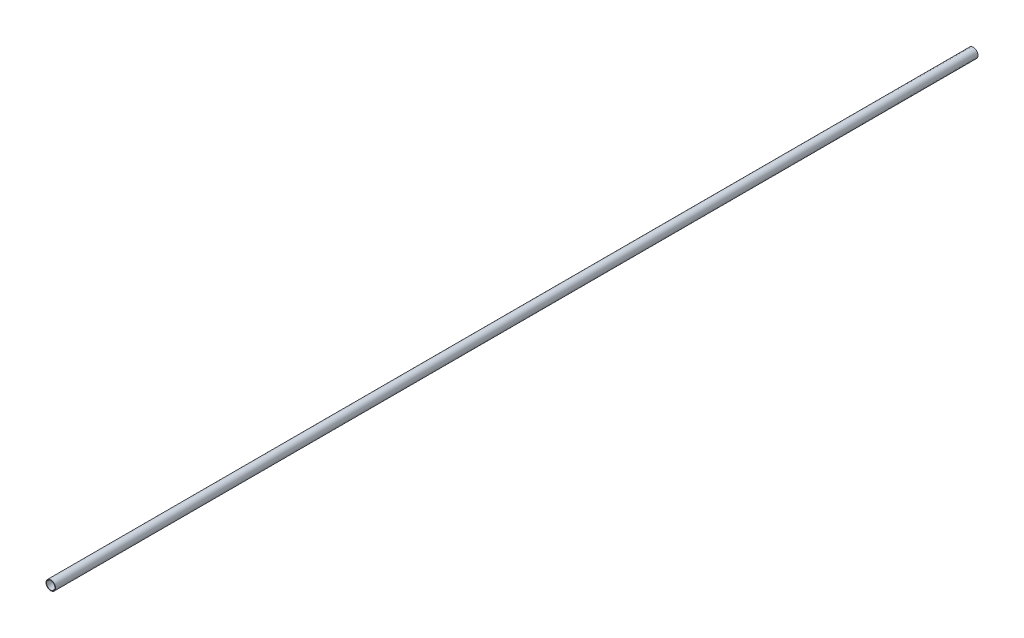
from build123d import *

# Parameters (mm, degrees)
SKETCH_1_R      = 16
SKETCH_1_R_2    = 14
EXTRUDE_1_DEPTH = 1550


with BuildPart() as part:
    # 草图1 → 凸台-拉伸1 (new, symmetric)
    with BuildSketch(Plane.XY):
        Circle(SKETCH_1_R)
        Circle(SKETCH_1_R_2, mode=Mode.SUBTRACT)
    extrude(amount=EXTRUDE_1_DEPTH, both=True)


solid = part.part
